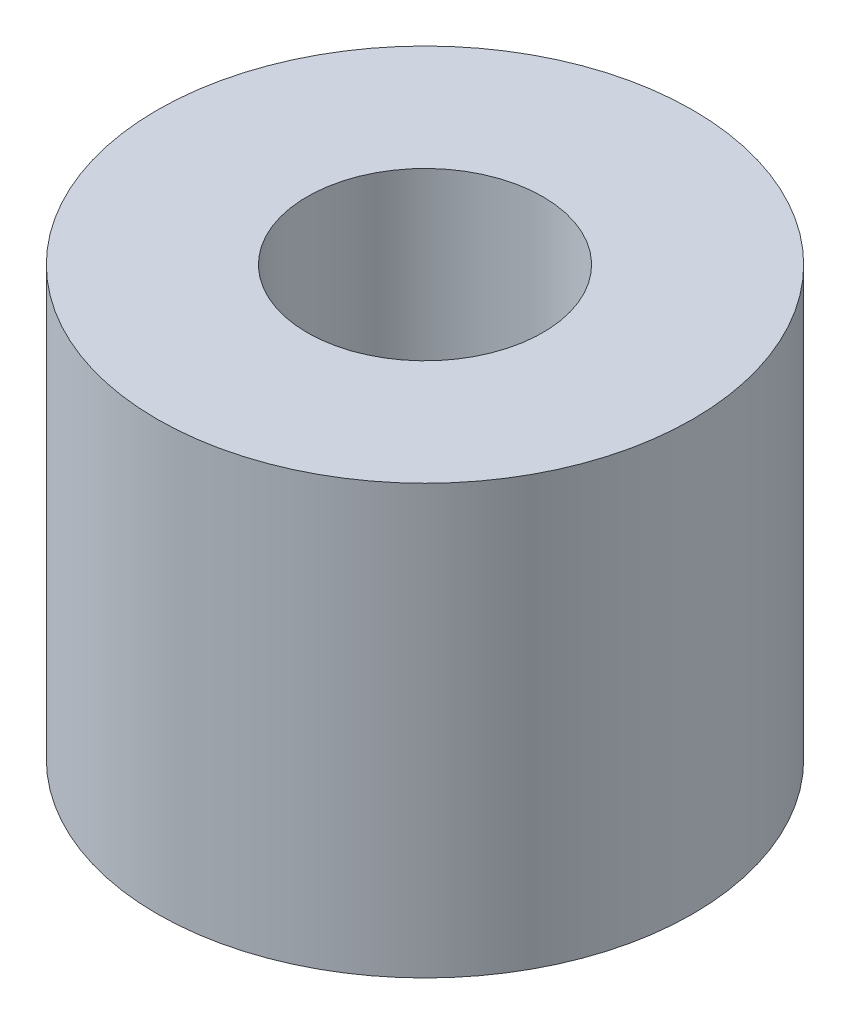
from build123d import *

# Parameters (mm, degrees)
SKETCH_1_R                   = 12.5
EXTRUDE_1_DEPTH              = 20
HOLE_WIZARD_M6_1_D           = 6.6
HOLE_WIZARD_M6_1_CBORE_D     = 11
HOLE_WIZARD_M6_1_CBORE_DEPTH = 10.8


with BuildPart() as part:
    # 草图1 → 凸台-拉伸1 (new body)
    with BuildSketch(Plane(origin=(0, 0, 0), x_dir=(1, 0, 0), z_dir=(0, 1, 0))):
        with Locations(Location((0, 0, 0), (0, 0, 270))):
            Circle(SKETCH_1_R)
    extrude(amount=EXTRUDE_1_DEPTH)

    # M6 六角圆柱头螺钉的柱形沉头孔1 (through all)
    with Locations(Plane(origin=(0, 20, 0), x_dir=(1, 0, 0), z_dir=(0, 1, 0))):
        with Locations((0, 0)):
            CounterBoreHole(HOLE_WIZARD_M6_1_D / 2, HOLE_WIZARD_M6_1_CBORE_D / 2, HOLE_WIZARD_M6_1_CBORE_DEPTH)


solid = part.part
